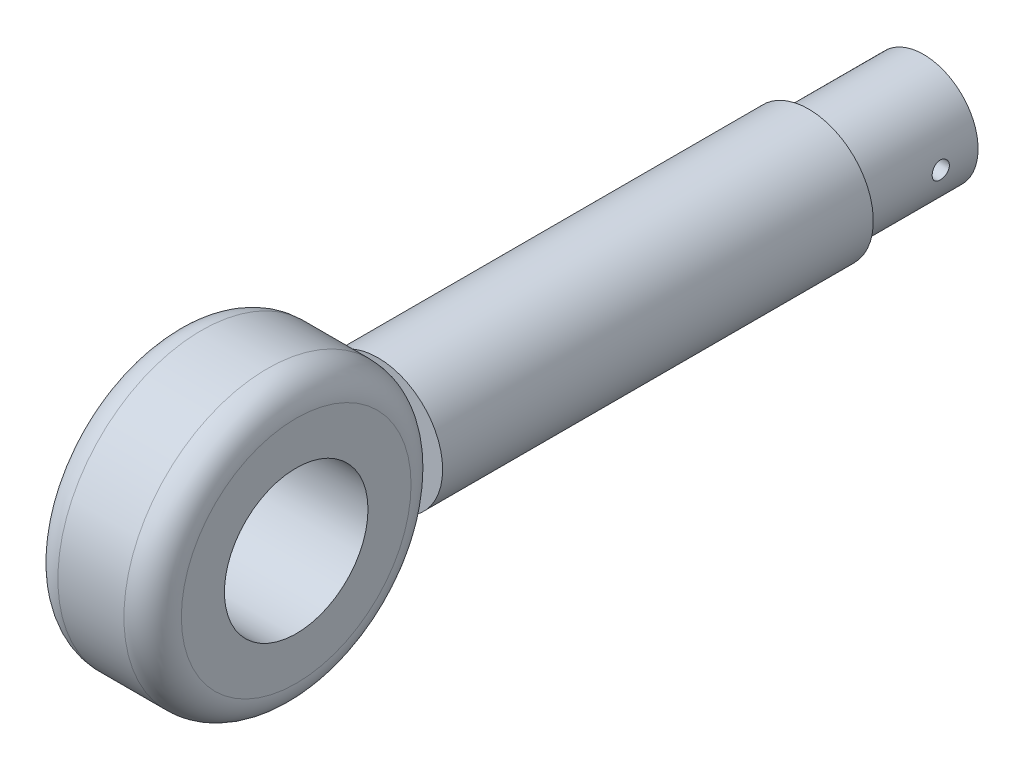
from build123d import *

# Parameters (mm, degrees)
SKETCH_1_R          = 22.5
EXTRUDE_1_DEPTH     = 190
SKETCH_2_R          = 50
SKETCH_2_R_2        = 25
EXTRUDE_2_DEPTH     = 21.5
FILLET_1_R          = 10
SKETCH_3_R          = 22.5
SKETCH_3_R_2        = 19
CUT_EXTRUDE_1_DEPTH = 40
SKETCH_4_R          = 3
CUT_EXTRUDE_2_DEPTH = 25


with BuildPart() as part:
    # 草图1 → 凸台-拉伸1 (new body)
    with BuildSketch(Plane.XY):
        Circle(SKETCH_1_R)
    extrude(amount=EXTRUDE_1_DEPTH)

    # 草图3 → 切除-拉伸1 (cut)
    with BuildSketch(Plane(origin=(0, 0, 0), x_dir=(-1, 0, 0), z_dir=(0, 0, -1))):
        Circle(SKETCH_3_R)
        Circle(SKETCH_3_R_2, mode=Mode.SUBTRACT)
    extrude(amount=-CUT_EXTRUDE_1_DEPTH, mode=Mode.SUBTRACT)

    # 草图4 → 切除-拉伸2 (cut, symmetric)
    with BuildSketch(Plane(origin=(0, 0, 0), x_dir=(0, 0, -1), z_dir=(1, 0, 0))):
        with Locations((-13, 0)):
            Circle(SKETCH_4_R)
    extrude(amount=CUT_EXTRUDE_2_DEPTH, both=True, mode=Mode.SUBTRACT)


with BuildPart() as body_2:
    # 草图2 → 凸台-拉伸2 (new, symmetric)
    with BuildSketch(Plane(origin=(0, 0, 0), x_dir=(0, 0, -1), z_dir=(1, 0, 0))):
        with Locations((-240, 0)):
            Circle(SKETCH_2_R)
        with Locations((-240, 0)):
            Circle(SKETCH_2_R_2, mode=Mode.SUBTRACT)
    extrude(amount=EXTRUDE_2_DEPTH, both=True)

    # 圆角1
    fillet_1_edges = [body_2.edges().sort_by_distance(p)[0] for p in [
        (-21.5, 0, 290),
        (21.5, 0, 290),
    ]]
    fillet(fillet_1_edges, radius=FILLET_1_R)


solid = Compound([part.part, body_2.part])
